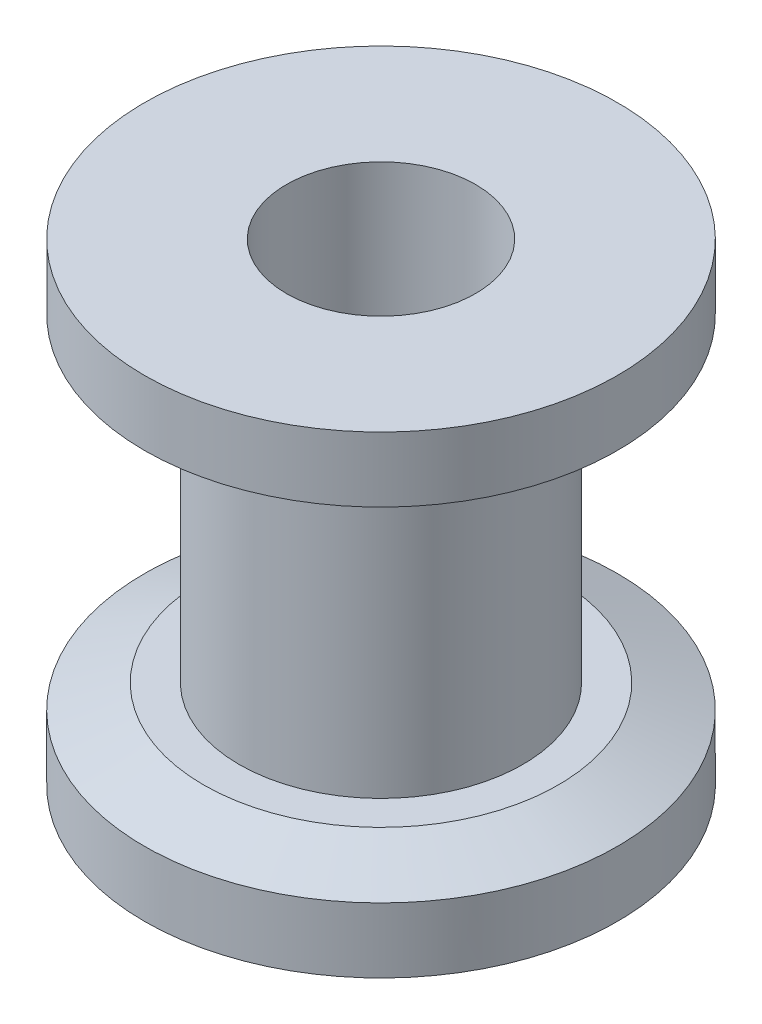
from build123d import *
from OCP.BRepFilletAPI import BRepFilletAPI_MakeChamfer

# Parameters (mm, degrees)
SKETCH1_R           = 20
SKETCH1_R_2         = 8
BOSS_EXTRUDE1_DEPTH = 40
SKETCH2_W           = 16
SKETCH2_H           = 25
CHAMFER1_SIZE       = 5
CHAMFER1_SIZE2      = 2


with BuildPart() as part:
    # Sketch1 → Boss-Extrude1 (new body)
    with BuildSketch(Plane(origin=(0, 0, 0), x_dir=(1, 0, 0), z_dir=(0, 1, 0))):
        with Locations(Location((0, 0, 0), (0, 0, 270))):
            Circle(SKETCH1_R)
        with Locations(Location((0, 0, 0), (0, 0, 270))):
            Circle(SKETCH1_R_2, mode=Mode.SUBTRACT)
    extrude(amount=BOSS_EXTRUDE1_DEPTH)

    # Sketch2 → Cut-Revolve1 (revolve, cut)
    with BuildSketch(Plane.XY, mode=Mode.PRIVATE) as cut_revolve1_sk:
        with Locations((20, 20)):
            Rectangle(SKETCH2_W, SKETCH2_H)
    revolve(cut_revolve1_sk.sketch.rotate(Axis((0, 0, 0), (0, 1, 0)), 90), axis=Axis((0, 0, 0), (0, 1, 0)), mode=Mode.SUBTRACT)

    # Chamfer1: one chamfer whose edges measure the first distance from different faces: ONE call of the kernel's chamfer builder (chamfer() names one face for all edges)
    chamfer1_edges_1 = [part.edges().sort_by_distance(p)[0] for p in [
        (0, 7.5, -20),
    ]]
    chamfer1_side_1 = [part.faces().sort_by_distance(p)[0] for p in [
        (0, 7.5, -19.434314575),
    ]]
    chamfer1_edges_2 = [part.edges().sort_by_distance(p)[0] for p in [
        (0, 32.5, -20),
    ]]
    chamfer1_side_2 = [part.faces().sort_by_distance(p)[0] for p in [
        (0, 32.5, -19.434314575),
    ]]
    chamfer1 = BRepFilletAPI_MakeChamfer(part.part.solid().wrapped)
    for e in chamfer1_edges_1:
        chamfer1.Add(CHAMFER1_SIZE, CHAMFER1_SIZE2, e.wrapped, chamfer1_side_1[0].wrapped)  # the first distance lies on this face
    for e in chamfer1_edges_2:
        chamfer1.Add(CHAMFER1_SIZE, CHAMFER1_SIZE2, e.wrapped, chamfer1_side_2[0].wrapped)  # the first distance lies on this face
    add(Compound.cast(chamfer1.Shape()), mode=Mode.REPLACE)


solid = part.part
